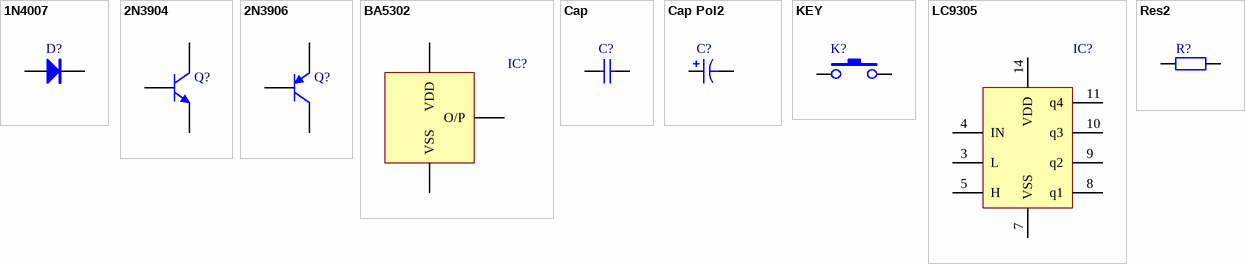
[diagram p0: symbols 1N4007 to Res2]
# Altium schematic symbol library MISC80621-6.SCHLIB: 9 symbols
Pins are listed as number, name and electrical type; pins without a type are passive.


## 1N4007
designator D?
Rectifier diode
footprint DO-41 (2.6*9.1mm (diameter, lead pitch))
footprint SOD-123 (2.7x1.6X1.1mm (length x width x height, excluding leads))
footprint SMA (4.5x2.6*2.2mm (length x width x height, excluding leads))
footprint DO-41V (2.6*3.5mm (diameter, lead pitch))
pins: 1 A, 2 K

## 2N3904
designator Q?
NPN General Purpose Amplifier
footprint TO-92A (TO, Flat Index; 3 In-Line, Axial Leads; Body Dia. 4.5mm; Leads 0.51 x 0.48 mm (max))
simulation model 2N3904 (NPN)
signal-integrity model 2N3904
pins: 1 E, 2 B, 3 C

## 2N3906
designator Q?
PNP General Purpose Amplifier
footprint TO-92A (TO, Flat Index; 3 In-Line, Axial Leads; Body Dia. 4.5mm; Leads 0.51 x 0.48 mm (max))
simulation model 2N3906 (PNP)
signal-integrity model 2N3906
pins: 1 E, 2 B, 3 C

## BA5302
designator IC?
footprint HDR1X3 (Connector; Header; 3 Position)
pins: 1 VDD, 2 O/P, 3 VSS

## Cap
designator C?
Capacitor
footprint RAD-0.3 (Radial Cap, Thru-Hole; 2 Leads; 0.3 in Pin Spacing)
simulation model CAP (Capacitor)
signal-integrity model Cap
pins: 1, 2

## Cap Pol2
designator C?
Polarized Capacitor (Axial)
footprint POLAR0.8 (Polarized Capacitor; 2 Leads)
simulation model CAP (Capacitor)
signal-integrity model Cap Pol
pins: 1, 2
1 alternate drawing of the same symbol

## KEY
designator K?
footprint DIP-3X6X4.3
footprint DIP-3X6X4.3_C
footprint DIP-3X6X5
footprint DIP-3X6X5_C
footprint DIP-6X6X4.3
footprint DIP-6X6X4.3_C
footprint DIP-6X6X5
footprint DIP-6X6X5_C
footprint DIP-6X6X5_C
footprint DIP-6X6X6
footprint DIP-6X6X6_C
footprint DIP-6X6X7
footprint DIP-6X6X7_C
footprint DIP-6X6X8
footprint DIP-6X6X8_C
footprint DIP-6X6X9
footprint DIP-6X6X9_C
footprint DIP-6X6X10
footprint DIP-6X6X10_C
footprint DIP-6X6X11
footprint DIP-6X6X11_C
footprint DIP-6X6X12
footprint DIP-6X6X12_C
footprint DIP-6X6X13
footprint DIP-6X6X14 (6*6*14mm)
footprint DIP-6X6X15
footprint DIP-12X12X4.3
footprint DIP-12X12X5
footprint DIP-12X12X6
footprint DIP-12X12X8
footprint DIP-12X12X9
footprint DIP-12X12X10
footprint DIP-12X12X11
footprint DIP-12X12X12
footprint DIP-12X12X13
footprint SMD-3X6X2.5
footprint SMD-3X6X4.3
footprint SMD-3X6X5
footprint SMD-4X4X1.5
footprint SMD-6X6X4.3
footprint SMD-6X6X5
footprint SMD-6X6X6
footprint SMD-6X6X7
footprint SMD-6X6X8
footprint SMD-6X6X9
footprint SMD-6X6X10
footprint SMD-6X6X11
footprint SMD-6X6X12
footprint SMD-6X6X13 (6*6*13mm)
footprint SMD-6X6X14
footprint SMD-6X6X15
footprint SMD-12X12X4.3
footprint SMD-12X12X5
footprint SMD-12X12X6
footprint SMD-12X12X7
footprint SMD-12X12X8 (12*12*8mm)
footprint SMD-12X12X9
footprint SMD-12X12X10
footprint SMD-12X12X11
footprint SMD-12X12X12 (12*12*12mm)
footprint SMD-12X12X13
footprint SMD-SW2X4
pins: 1, 3

## LC9305
designator IC?
footprint DIP14
pins: 3 L, 4 IN, 5 H, 7 VSS, 8 q1, 9 q2, 10 q3, 11 q4, 14 VDD

## Res2
designator R?
Resistor
footprint AXIAL-0.4 (Axial Device, Thru-Hole; 2 Leads; 0.4 in Pin Spacing)
simulation model RESISTOR (Resistor)
signal-integrity model Res
pins: 1, 2